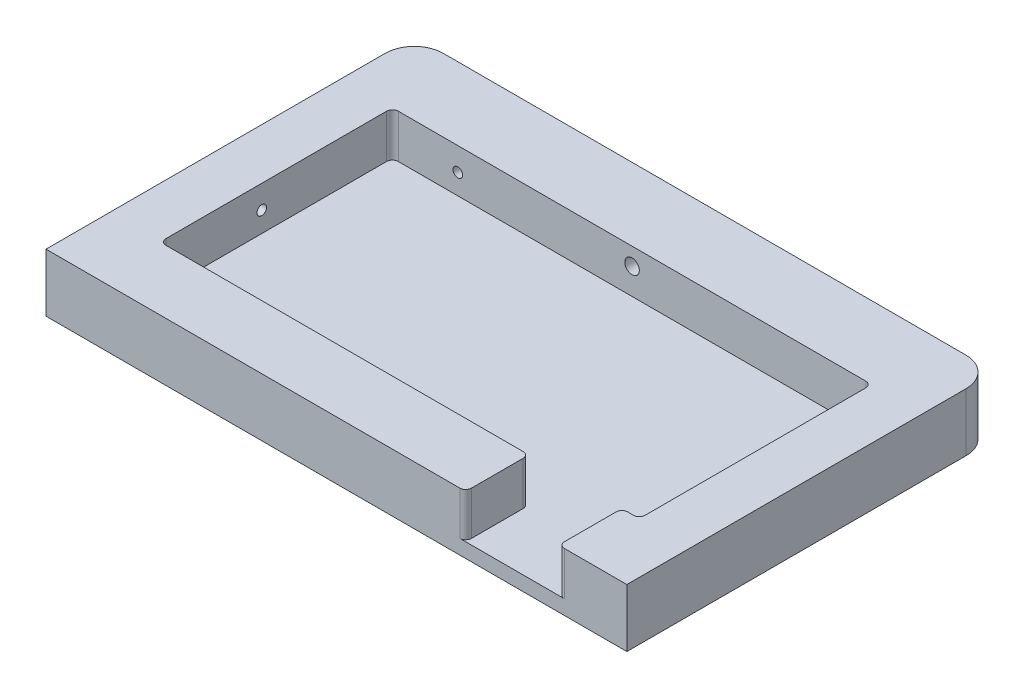
from build123d import *

# Parameters (mm, degrees)
SKETCH1_W             = 200
SKETCH1_H             = 150
BOSS_EXTRUDE1_DEPTH   = 20
SKETCH2_R             = 3
BOSS_EXTRUDE2_DEPTH   = 5
M6_TAPPED_HOLE1_D     = 5
M6_TAPPED_HOLE1_DEPTH = 25
M6_TAPPED_HOLE1_TIP   = 1.502151548
CUT_EXTRUDE1_DEPTH    = 15
SKETCH6_W             = 16
SKETCH6_H             = 15
CUT_EXTRUDE2_DEPTH    = 129.937969582
FILLET1_R             = 2
M4_TAPPED_HOLE1_D     = 3.3
M4_TAPPED_HOLE1_DEPTH = 30
M4_TAPPED_HOLE1_TIP   = 0.991420021
FILLET2_R             = 10
M4_TAPPED_HOLE2_D     = 3.3
M4_TAPPED_HOLE2_DEPTH = 30
M4_TAPPED_HOLE2_TIP   = 0.991420021
CUT_EXTRUDE3_DEPTH    = 130.614813968
FILLET3_R             = 2


with BuildPart() as part:
    # Sketch1 → Boss-Extrude1 (new body)
    with BuildSketch(Plane(origin=(0, 0, 0), x_dir=(1, 0, 0), z_dir=(0, 1, 0))):
        Rectangle(SKETCH1_W, SKETCH1_H)
    extrude(amount=BOSS_EXTRUDE1_DEPTH)

    # Sketch2 → Boss-Extrude2 (add)
    with BuildSketch(Plane(origin=(0, 0, -75), x_dir=(-1, 0, 0), z_dir=(0, 0, -1))):
        with Locations(Location((0, 5, 0), (0, 0, 180))):
            Circle(SKETCH2_R)
    extrude(amount=BOSS_EXTRUDE2_DEPTH)

    # M6 Tapped Hole1
    with Locations(Plane(origin=(0, 0, -75), x_dir=(-1, 0, 0), z_dir=(0, 0, -1))):
        with Locations((0, 14)):
            Hole(M6_TAPPED_HOLE1_D / 2, depth=M6_TAPPED_HOLE1_DEPTH)
            with Locations((0, 0, -(M6_TAPPED_HOLE1_DEPTH + M6_TAPPED_HOLE1_TIP / 2))):  # 118° drill point
                Cone(0, M6_TAPPED_HOLE1_D / 2, M6_TAPPED_HOLE1_TIP, mode=Mode.SUBTRACT)

    # Sketch5 → Cut-Extrude1 (cut)
    with BuildSketch(Plane(origin=(0, 20, 0), x_dir=(1, 0, 0), z_dir=(0, 1, 0))):
        Polygon((-82.5, 50), (44.5, 50), (76.5, 50), (82.5, 50), (82.5, -30), (76.5, -30), (76.5, -51.78814737), (68.5, -51.78814737), (68.5, -66.78814737), (52.5, -66.78814737), (52.5, -51.78814737), (44.5, -51.78814737), (44.5, -30), (-82.5, -30), align=None)
    extrude(amount=-CUT_EXTRUDE1_DEPTH, mode=Mode.SUBTRACT)

    # Sketch6 → Cut-Extrude2 (cut, through all)
    with BuildSketch(Plane(origin=(0, 5, 0), x_dir=(1, 0, 0), z_dir=(0, 1, 0))):
        with Locations((60.5, -59.28814737)):
            Rectangle(SKETCH6_W, SKETCH6_H)
    extrude(amount=-CUT_EXTRUDE2_DEPTH, mode=Mode.SUBTRACT)

    # Fillet1
    fillet1_edges = [part.edges().sort_by_distance(p)[0] for p in [
        (-82.5, 12.5, -50),
        (-82.5, 12.5, 30),
        (82.5, 12.5, -50),
        (82.5, 12.5, 30),
        (76.5, 12.5, 30),
        (68.5, 12.5, 51.78814737),
        (68.5, 10, 66.78814737),
        (52.5, 10, 66.78814737),
        (52.5, 12.5, 51.78814737),
        (44.5, 12.5, 30),
    ]]
    fillet(fillet1_edges, radius=FILLET1_R)

    # M4 Tapped Hole1
    with Locations(Plane.ZY.offset(100)):
        with Locations((-5, 12)):
            Hole(M4_TAPPED_HOLE1_D / 2, depth=M4_TAPPED_HOLE1_DEPTH)
            with Locations((0, 0, -(M4_TAPPED_HOLE1_DEPTH + M4_TAPPED_HOLE1_TIP / 2))):  # 118° drill point
                Cone(0, M4_TAPPED_HOLE1_D / 2, M4_TAPPED_HOLE1_TIP, mode=Mode.SUBTRACT)

    # Fillet2
    fillet2_edges = [part.edges().sort_by_distance(p)[0] for p in [
        (100, 10, 75),
        (-100, 10, 75),
        (-100, 10, -75),
        (100, 10, -75),
    ]]
    fillet(fillet2_edges, radius=FILLET2_R)

    # M4 Tapped Hole2
    with Locations(Plane(origin=(0, 0, -75), x_dir=(-1, 0, 0), z_dir=(0, 0, -1))):
        with Locations((60, 12)):
            Hole(M4_TAPPED_HOLE2_D / 2, depth=M4_TAPPED_HOLE2_DEPTH)
            with Locations((0, 0, -(M4_TAPPED_HOLE2_DEPTH + M4_TAPPED_HOLE2_TIP / 2))):  # 118° drill point
                Cone(0, M4_TAPPED_HOLE2_D / 2, M4_TAPPED_HOLE2_TIP, mode=Mode.SUBTRACT)

    # Sketch13 → Cut-Extrude3 (cut, through all)
    with BuildSketch(Plane(origin=(0, 20, 0), x_dir=(1, 0, 0), z_dir=(0, 1, 0))):
        Polygon((73.5, -51.78814737), (115.827704394, -51.78814737), (115.827704394, -85.085952347), (72.5, -85.085952347), (-109.048113532, -107.181271315), (-117.406351495, -51.78814737), align=None)
    extrude(amount=-CUT_EXTRUDE3_DEPTH, mode=Mode.SUBTRACT)

    # Fillet3
    fillet3_edges = [part.edges().sort_by_distance(p)[0] for p in [
        (76.5, 12.5, 51.78814737),
        (44.5, 12.5, 51.78814737),
    ]]
    fillet(fillet3_edges, radius=FILLET3_R)


solid = part.part
